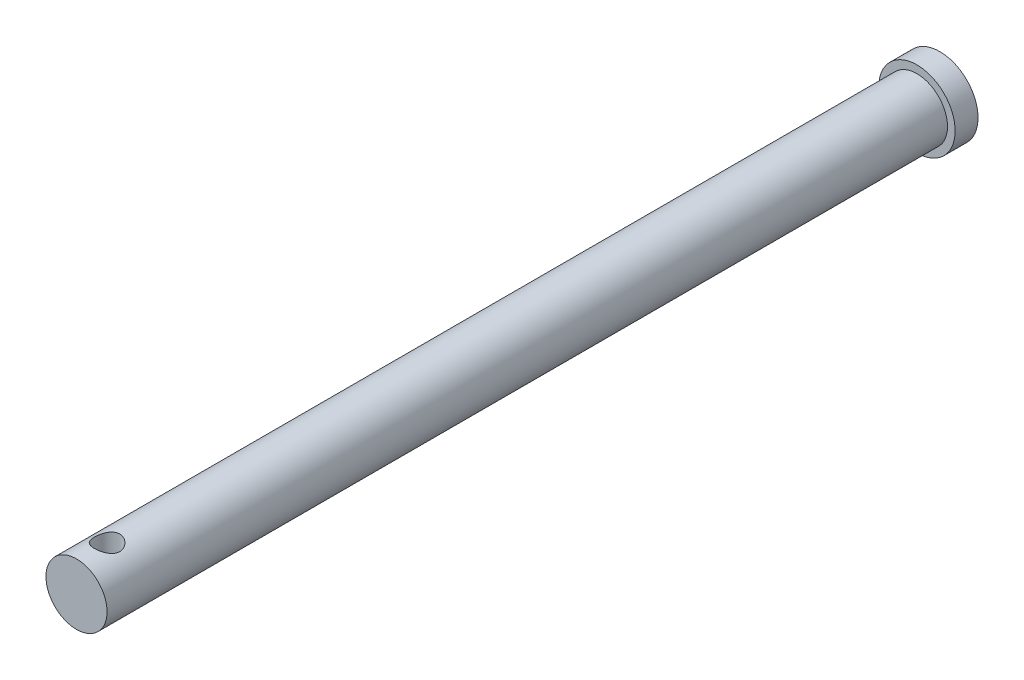
from build123d import *

# Parameters (mm, degrees)
SKETCH1_R           = 4
BOSS_EXTRUDE1_DEPTH = 110
SKETCH7_R           = 5
BOSS_EXTRUDE2_DEPTH = 3
SKETCH9_W           = 1.65
SKETCH9_H           = 5


with BuildPart() as part:
    # Sketch1 → Boss-Extrude1 (new body)
    with BuildSketch(Plane.XY):
        Circle(SKETCH1_R)
    extrude(amount=BOSS_EXTRUDE1_DEPTH)

    # Sketch7 → Boss-Extrude2 (add)
    with BuildSketch(Plane(origin=(0, 0, 0), x_dir=(-1, 0, 0), z_dir=(0, 0, -1))):
        Circle(SKETCH7_R)
    extrude(amount=BOSS_EXTRUDE2_DEPTH)

    # Sketch9 → M4 Tapped Hole1 (revolve, cut)
    with BuildSketch(Plane(origin=(0, 0, 106), x_dir=(0, 0, -1), z_dir=(1, 0, 0))):
        with Locations((0.825, 2.5)):
            Rectangle(SKETCH9_W, SKETCH9_H)
    revolve(axis=Axis((0, -6.35, 106), (0, 1, 0)), mode=Mode.SUBTRACT)


solid = part.part
